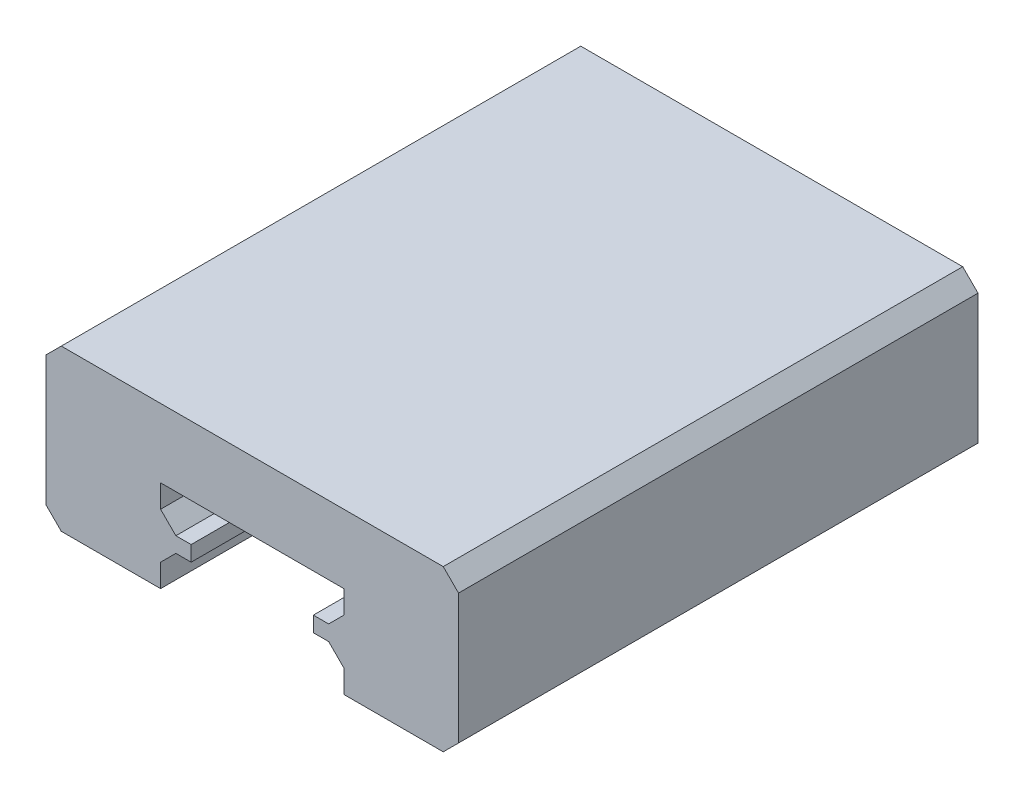
from build123d import *

# Parameters (mm, degrees)
BOSS_EXTRUDE1_DEPTH = 34
CHAMFER1_SIZE       = 1


with BuildPart() as part:
    # Sketch1 → Boss-Extrude1 (new body)
    with BuildSketch(Plane.XY):
        Polygon((-13.5, 5), (13.5, 5), (13.5, -5.5), (6, -5.5), (6, -4), (5, -3), (4, -3), (4, -2), (5, -2), (6, -1), (6, 0.5), (-6, 0.5), (-6, -1), (-5, -2), (-4, -2), (-4, -3), (-5, -3), (-6, -4), (-6, -5.5), (-13.5, -5.5), align=None)
    extrude(amount=BOSS_EXTRUDE1_DEPTH)

    # Chamfer1
    chamfer1_edges = [part.edges().sort_by_distance(p)[0] for p in [
        (-13.5, -5.5, 17),
        (-13.5, 5, 17),
        (13.5, 5, 17),
        (13.5, -5.5, 17),
    ]]
    chamfer(chamfer1_edges, length=CHAMFER1_SIZE)


solid = part.part
